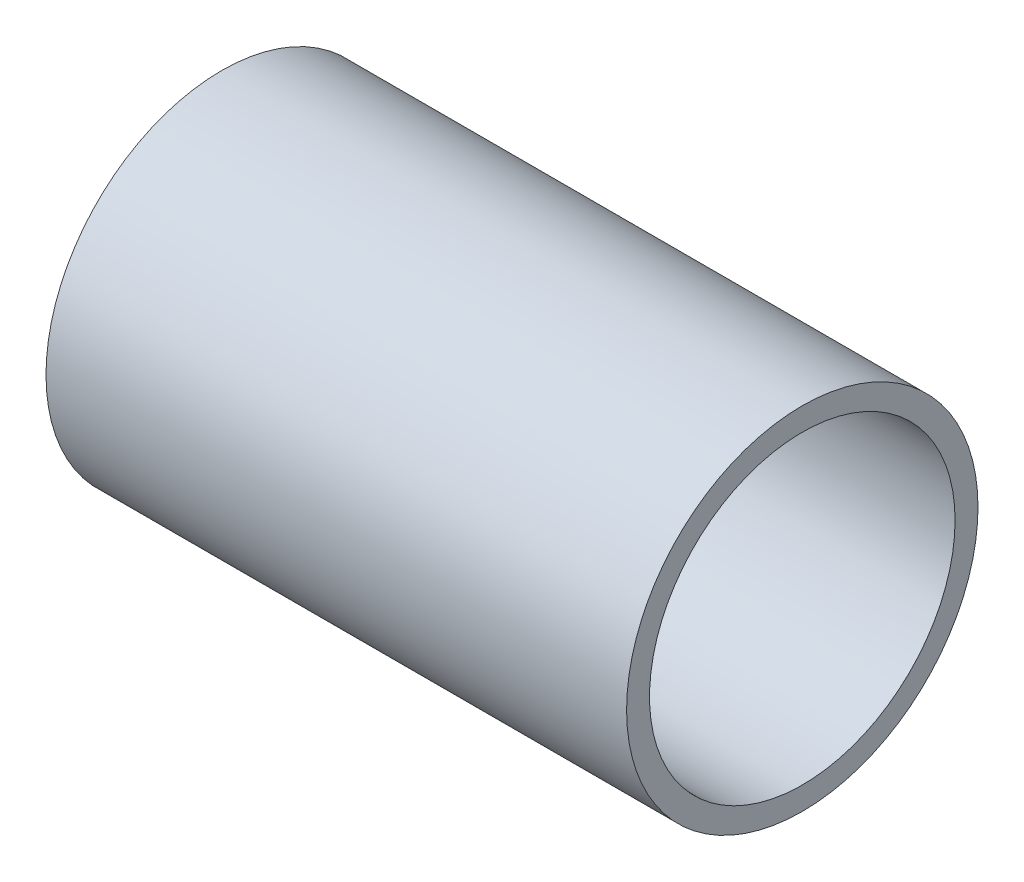
SolidWorks part; units mm, degrees
ref_plane "前视基准面" through (0, 0, 0) normal (0, 0, 1) x (1, 0, 0)
ref_plane "上视基准面" through (0, 0, 0) normal (0, 1, 0) x (1, 0, 0)
ref_plane "右视基准面" through (0, 0, 0) normal (1, 0, 0) x (0, 0, -1)
sketch "草图1" plane through (0, 0, 0) normal (1, 0, 0) x (0, 0, -1)
  circle A0 centre (0, 0) radius 20
  circle A1 centre (0, 0) radius 23
extrude "凸台-拉伸1" add sketch "草图1" along normal blind 76
